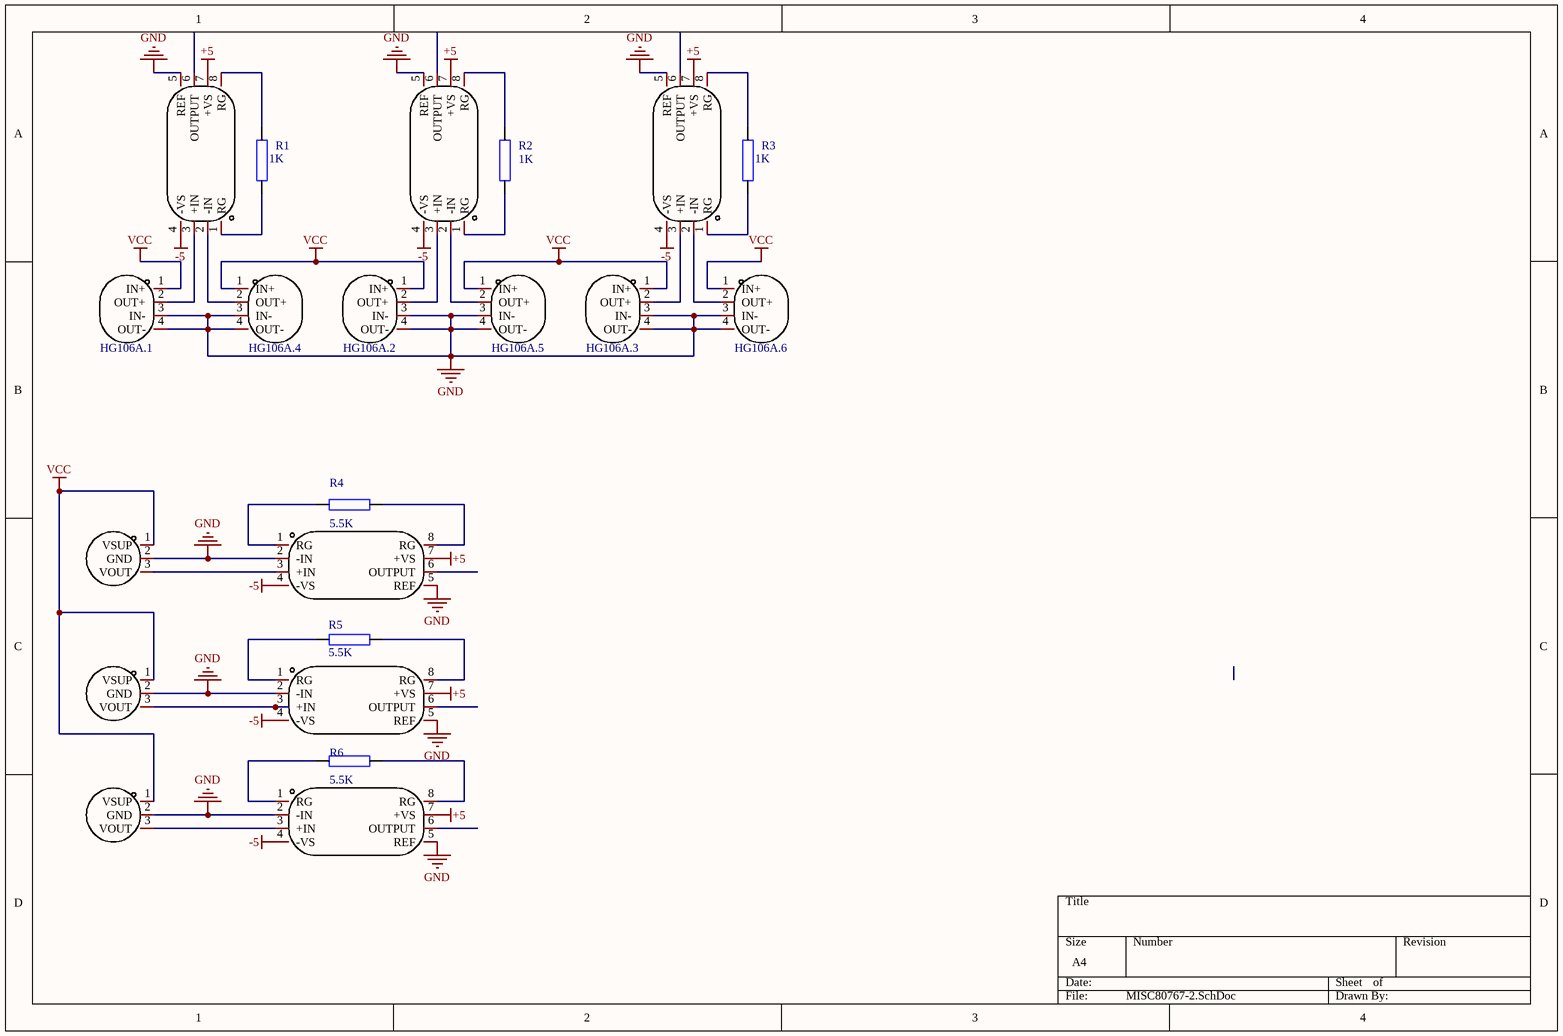
[diagram p0: MISC80767-2.SchDoc]
# Altium project MISC80767-3.PrjPcb
1 sheet, 21 parts. Net scope: global (net labels, ports and power ports of the same name join across sheets).
Board file: MISC80767.PcbDoc

## Sheet MISC80767-2.SchDoc
size A4; SheetNumber: 1; SheetTotal: 1

### Parts
R1  1K  [R一般电阻/10mm]
R2  1K  [R一般电阻/10mm]
R3  1K  [R一般电阻/10mm]
R4  5.5K  [R一般电阻/10mm]
R5  5.5K  [R一般电阻/10mm]
R6  5.5K  [R一般电阻/10mm]
U1  AD620ARZ-REEL  [SOIC-8_L5.0-W4.0-P1.27-LS6.0-BL]  (value not drawn)
U2  AD620ARZ-REEL  [SOIC-8_L5.0-W4.0-P1.27-LS6.0-BL]  (value not drawn)
U3  AD620ARZ-REEL  [SOIC-8_L5.0-W4.0-P1.27-LS6.0-BL]  (value not drawn)
U4  HG106A  [SOP-4_L1.5-W1.5-P0.90-LS2.5-BL]  (value not drawn)
U5  HG106A  [SOP-4_L1.5-W1.5-P0.90-LS2.5-BL]  (value not drawn)
U6  HG106A  [SOP-4_L1.5-W1.5-P0.90-LS2.5-BL]  (value not drawn)
U7  HG106A  [SOP-4_L1.5-W1.5-P0.90-LS2.5-BL]  (value not drawn)
U8  HG106A  [SOP-4_L1.5-W1.5-P0.90-LS2.5-BL]  (value not drawn)
U9  HG106A  [SOP-4_L1.5-W1.5-P0.90-LS2.5-BL]  (value not drawn)
U10  JSM3144  [SOT-23-3_L2.9-W1.6-P1.90-LS2.8-BR-CW]  (value not drawn)
U11  AD620ARZ-REEL  [SOIC-8_L5.0-W4.0-P1.27-LS6.0-BL]  (value not drawn)
U12  JSM3144  [SOT-23-3_L2.9-W1.6-P1.90-LS2.8-BR-CW]  (value not drawn)
U13  AD620ARZ-REEL  [SOIC-8_L5.0-W4.0-P1.27-LS6.0-BL]  (value not drawn)
U14  JSM3144  [SOT-23-3_L2.9-W1.6-P1.90-LS2.8-BR-CW]  (value not drawn)
U15  AD620ARZ-REEL  [SOIC-8_L5.0-W4.0-P1.27-LS6.0-BL]  (value not drawn)

### Nets
+5: U1.7(+VS) U2.7(+VS) U3.7(+VS) U11.7(+VS) U13.7(+VS) U15.7(+VS)
-5: U1.4(-VS) U2.4(-VS) U3.4(-VS) U11.4(-VS) U13.4(-VS) U15.4(-VS)
GND: U1.5(REF) U2.5(REF) U3.5(REF) U4.3(IN-) U4.4(OUT-) U5.3(IN-) U5.4(OUT-) U6.3(IN-) U6.4(OUT-) U7.3(IN-) U7.4(OUT-) U8.3(IN-) U8.4(OUT-) U9.3(IN-) U9.4(OUT-) U10.2(GND) U11.2(-IN) U11.5(REF) U12.2(GND) U13.2(-IN) U13.5(REF) U14.2(GND) U15.2(-IN) U15.5(REF)
VCC: U4.1(IN+) U5.1(IN+) U6.1(IN+) U7.1(IN+) U8.1(IN+) U9.1(IN+) U10.1(VSUP) U12.1(VSUP) U14.1(VSUP)
NetR1_1: R1.1 U1.1(RG)
NetR1_2: R1.2 U1.8(RG)
NetR2_1: R2.1 U2.1(RG)
NetR2_2: R2.2 U2.8(RG)
NetR3_1: R3.1 U3.1(RG)
NetR3_2: R3.2 U3.8(RG)
NetR4_1: R4.1 U11.8(RG)
NetR4_2: R4.2 U11.1(RG)
NetR5_1: R5.1 U13.8(RG)
NetR5_2: R5.2 U13.1(RG)
NetR6_1: R6.1 U15.8(RG)
NetR6_2: R6.2 U15.1(RG)
NetU1_2: U1.2(-IN) U5.2(OUT+)
NetU1_3: U1.3(+IN) U4.2(OUT+)
NetU2_2: U2.2(-IN) U7.2(OUT+)
NetU2_3: U2.3(+IN) U6.2(OUT+)
NetU3_2: U3.2(-IN) U9.2(OUT+)
NetU3_3: U3.3(+IN) U8.2(OUT+)
NetU10_3: U10.3(VOUT) U11.3(+IN)
NetU12_3: U12.3(VOUT) U13.3(+IN)
NetU14_3: U14.3(VOUT) U15.3(+IN)

Not connected (* = marked no-connect by the designer): U1 6(OUTPUT); U2 6(OUTPUT); U3 6(OUTPUT); U11 6(OUTPUT); U13 6(OUTPUT); U15 6(OUTPUT)

### Notes on the sheet
- (near U4) HG106A.1
- (near U5) HG106A.4
- (near U6) HG106A.2
- (near U7) HG106A.5
- (near U8) HG106A.3
- (near U9) HG106A.6

### Library data of the parts
R1-R6 = R一般电阻
U1-U3 U11 U13 U15 = AD620ARZ-REEL: Manufacturer: ADI(亚德诺); Symbol: AD620ARZ-REEL_C253558; Add into BOM: yes; Number of Circuits: parameter Number of Circuits single-channel; Current - Input Bias(Ib): 500pA; Voltage - Input Offset(Vos): 30uV; Slew Rate(SR): 1.2V/us; -3db Bandwidth: 1MHz; Device: AD620ARZ-REEL; LCSC Part Name: 低成本、低功耗仪表放大器; Supplier Part: C253558; Manufacturer Part: AD620ARZ-REEL; Supplier Footprint: SOIC-8; JLCPCB Part Class: Extended Part; Datasheet: parameter Datasheet text  https://example.com/upload/public/pdf/source/20180712/C253558_3CD382589248680FDE910573D3ACFCEF.pdf; Supplier: LCSC; Convert to PCB: yes; Gain Bandwidth Product(GBP): -; Operating Temperature: -40℃~+85℃
U4-U9 = HG106A_1: Manufacturer: AKM; Add into BOM: yes; supply voltage: 8V; Symbol: HG106A; Device: HG106A; LCSC Part Name: HG106A; Supplier Part: C3716218; Manufacturer Part: HG106A; Supplier Footprint: SOP-4; JLCPCB Part Class: Extended Part; Datasheet: parameter Datasheet text  https://example.com/upload/public/pdf/source/20240124/CC8B0D81688B28624AA92D542C2D4D83.pdf; Supplier: LCSC; Convert to PCB: yes; Operating Temperature: -40℃~+125℃
U10 U12 U14 = JSM3144: Manufacturer: JSMSEMI(杰盛微); Add into BOM: yes; supply voltage: 3.8V~40V; Symbol: JSM3144; Device: JSM3144; LCSC Part Name: 单极霍尔开关; Supplier Part: C2900615; Manufacturer Part: JSM3144; Supplier Footprint: SOT-23; JLCPCB Part Class: Extended Part; Datasheet: parameter Datasheet text  https://example.com/upload/public/pdf/source/20240105/E9D95608E1A6A7F9F4DCAC757C11DCFA.pdf; Supplier: LCSC; Convert to PCB: yes; Operating Temperature: -40℃~+125℃